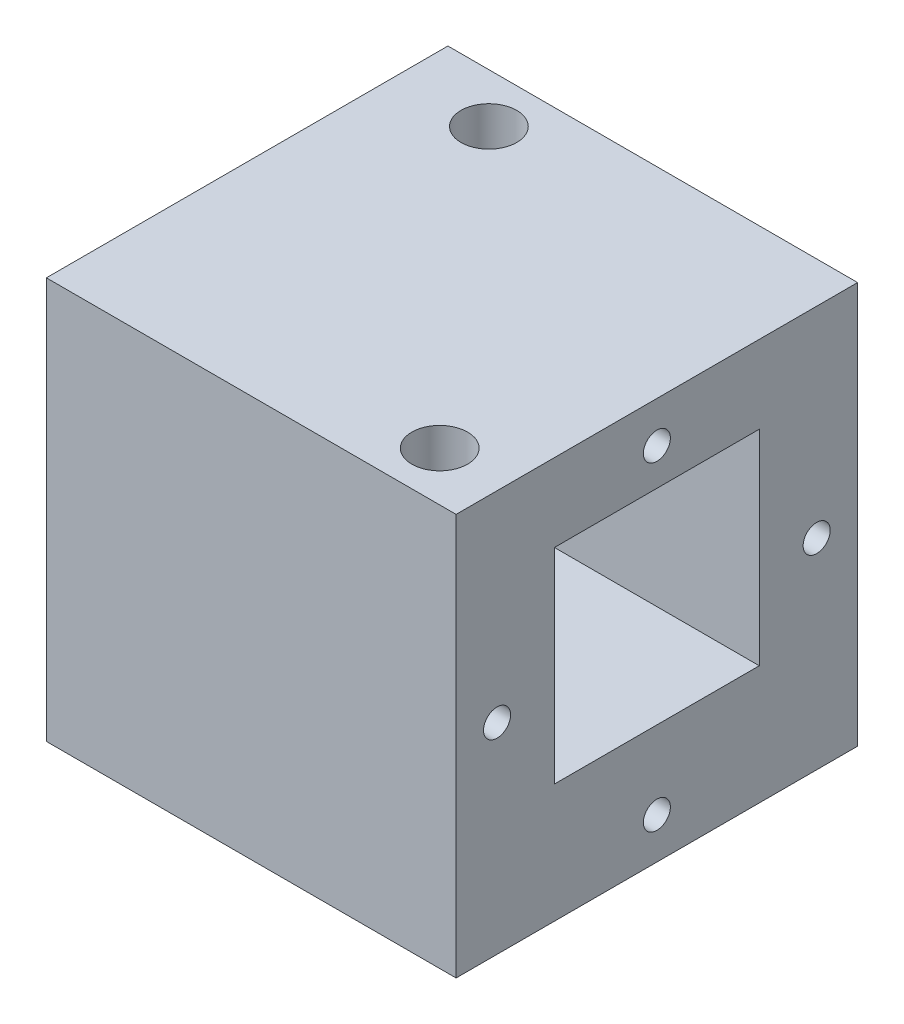
from build123d import *

# Parameters (mm, degrees)
SKETCH_2_W             = 49
SKETCH_2_H             = 49
EXTRUDE_2_DEPTH        = 50
SKETCH_3_W             = 25
SKETCH_3_H             = 25
CUT_EXTRUDE_1_DEPTH    = 50
HOLE_WIZARD_M4_1_D     = 3.3
HOLE_WIZARD_M4_1_DEPTH = 13.5
HOLE_WIZARD_M4_1_TIP   = 0.991420021
HOLE_WIZARD_M8_1_D     = 6.8
HOLE_WIZARD_M8_1_DEPTH = 18
HOLE_WIZARD_M8_1_TIP   = 2.042926105


with BuildPart() as part:
    # 草图2 → 凸台-拉伸2 (new body)
    with BuildSketch(Plane(origin=(0, 0, 0), x_dir=(0, 0, -1), z_dir=(1, 0, 0))):
        with Locations((24.5, 24.5)):
            Rectangle(SKETCH_2_W, SKETCH_2_H)
    extrude(amount=EXTRUDE_2_DEPTH)

    # 草图3 → 切除-拉伸1 (cut)
    with BuildSketch(Plane(origin=(50, 0, 0), x_dir=(0, 0, -1), z_dir=(1, 0, 0))):
        with Locations((24.5, 27)):
            Rectangle(SKETCH_3_W, SKETCH_3_H)
    extrude(amount=-CUT_EXTRUDE_1_DEPTH, mode=Mode.SUBTRACT)

    # M4 螺纹孔1
    with Locations(Plane(origin=(50, 0, 0), x_dir=(0, 0, -1), z_dir=(1, 0, 0))):
        with Locations((24.5, 44), (5, 24.5), (24.5, 5), (44, 24.5)):
            Hole(HOLE_WIZARD_M4_1_D / 2, depth=HOLE_WIZARD_M4_1_DEPTH)
            with Locations((0, 0, -(HOLE_WIZARD_M4_1_DEPTH + HOLE_WIZARD_M4_1_TIP / 2))):  # 118° drill point
                Cone(0, HOLE_WIZARD_M4_1_D / 2, HOLE_WIZARD_M4_1_TIP, mode=Mode.SUBTRACT)

    # M8 螺纹孔1
    with Locations(Plane(origin=(0, 49, 0), x_dir=(-1, 0, 0), z_dir=(0, 1, 0))):
        with Locations((-42, -6), (-11, -43)):
            Hole(HOLE_WIZARD_M8_1_D / 2, depth=HOLE_WIZARD_M8_1_DEPTH)
            with Locations((0, 0, -(HOLE_WIZARD_M8_1_DEPTH + HOLE_WIZARD_M8_1_TIP / 2))):  # 118° drill point
                Cone(0, HOLE_WIZARD_M8_1_D / 2, HOLE_WIZARD_M8_1_TIP, mode=Mode.SUBTRACT)


solid = part.part
